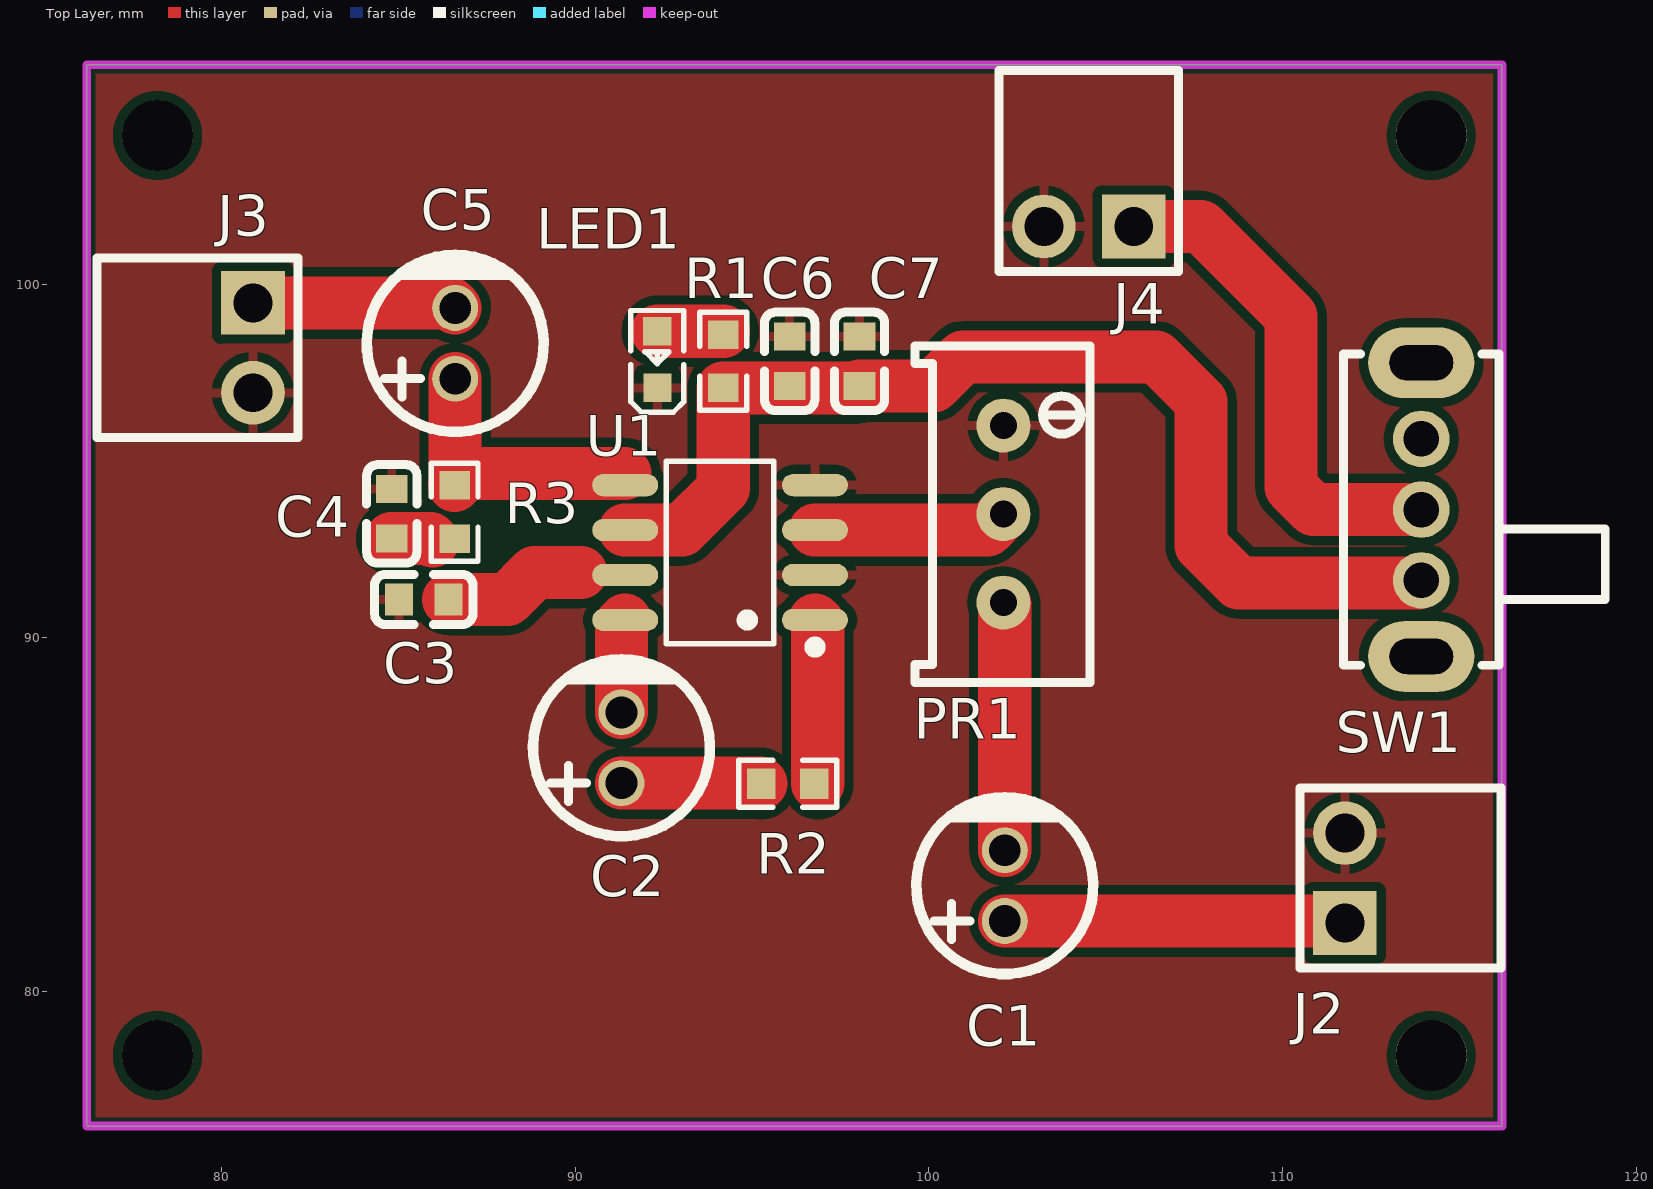
[diagram p0: Top Layer view]
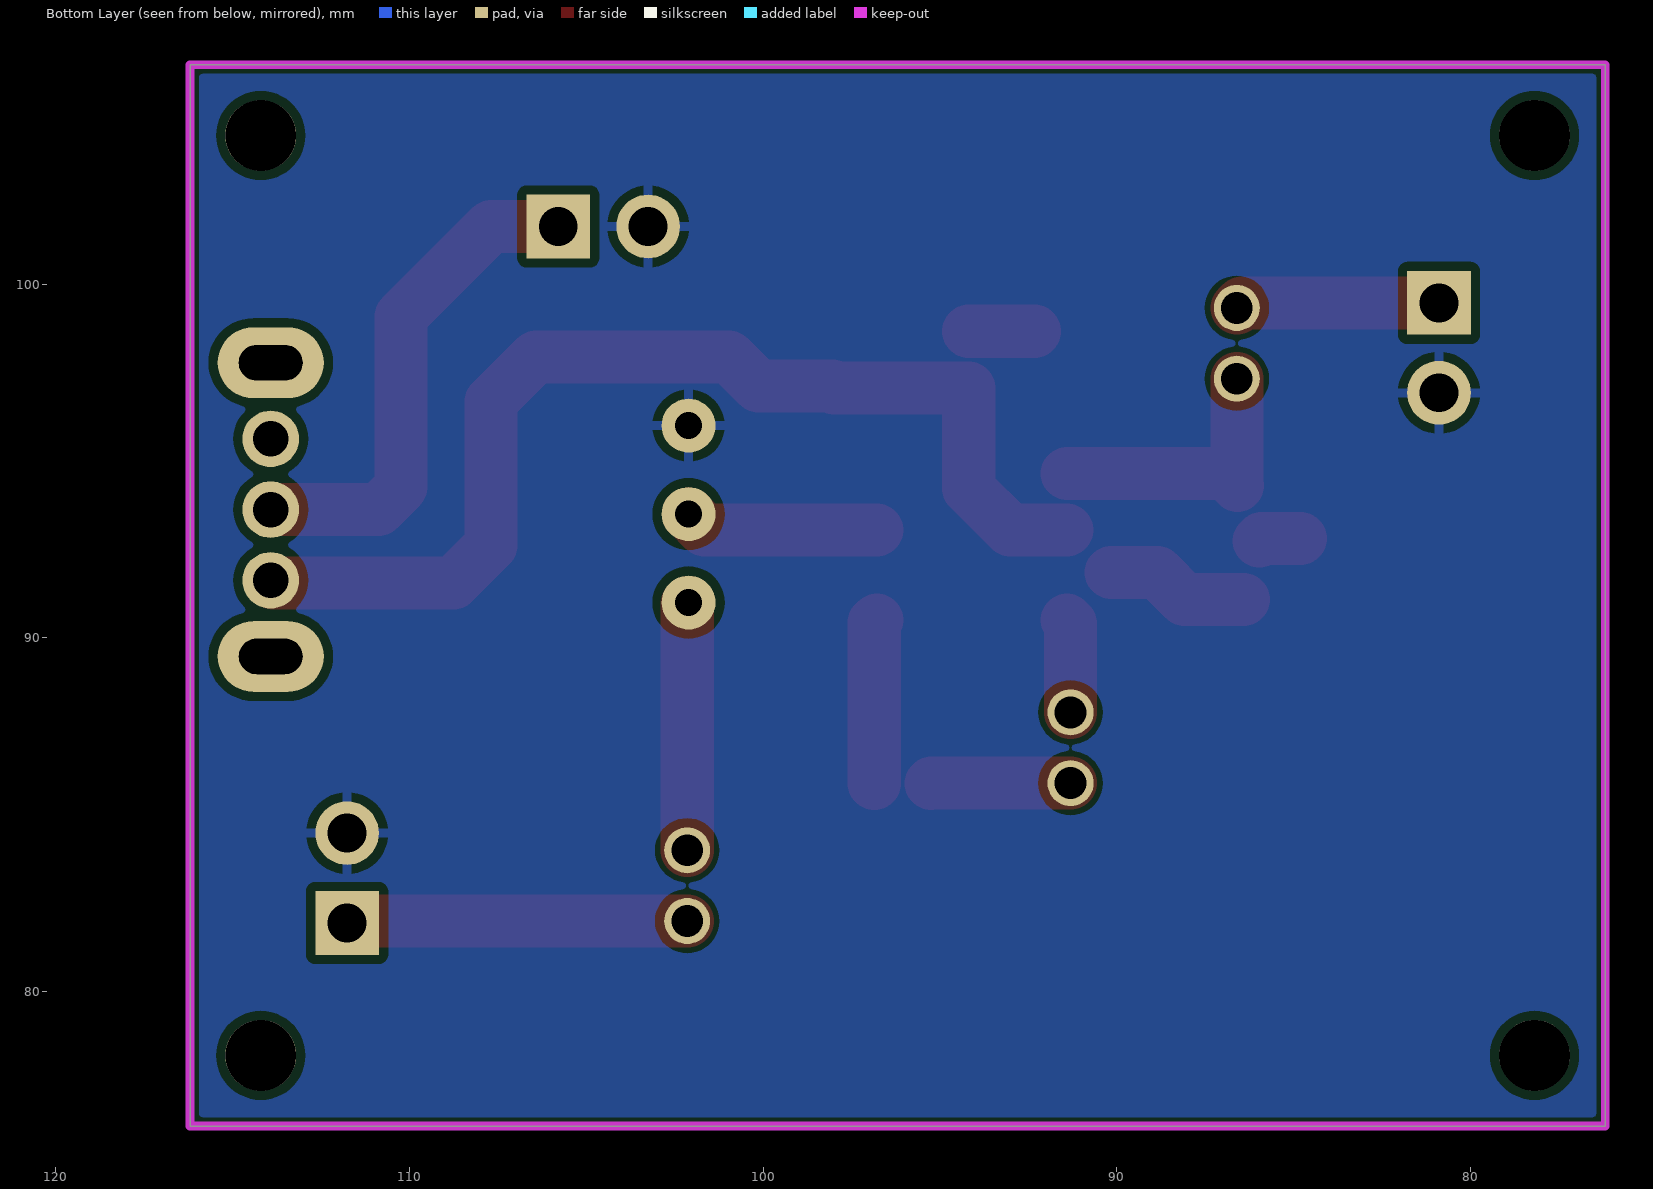
[diagram p1: Bottom Layer view, seen from below]
# Altium PCB MISC52147.pcbdoc
Units mm, origin at the board's own origin, x right, y up, seen from the top; angles counter-clockwise.
Board outline 40 x 30 mm, 2 copper layers (Top Layer, Bottom Layer), stack 1.58 mm thick; 17 components, 14 nets, 48 pads, 0 vias.

## Layer stack, top to bottom
Top Solder Mask Layer: solder mask 0.01, Dk 3.3
Top Layer: signal copper 0.035
Dielectric1: surface 1.51, FR4, Dk 4.5
Bottom Layer: signal copper 0.035
Bottom Solder Mask Layer: solder mask 0.01, Dk 3.3

## Board outline
76.2,106.2 76.2,76.2 116.2,76.2 116.2,106.2

## Design rules (kind name [scope] priority, off if disabled: settings)
BoardOutlineClearance copperThickness2oz_1 [All] p2 off: genericclearance=0.203 ignorepadtopadclearanceinfootprint=FALSE except(0: Arc-SplitContinuation Track-SplitContinuation SMDPad-SplitContinuation THPad-SplitContinuation Via-SplitContinuation Fill-SplitContinuation Region-SplitContinuation Poly-SplitContinuation Text-SplitContinuation Hole-SplitContinuation; 0.152: Arc-CutoutEdge SMDPad-CutoutEdge THPad-CutoutEdge Via-CutoutEdge Fill-CutoutEdge Region-CutoutEdge Text-CutoutEdge; 0.176: Hole-OutlineEdge Hole-CutoutEdge; 0.254: Poly-OutlineEdge Poly-CutoutEdge; 0.3: Arc-OutlineEdge Track-OutlineEdge SMDPad-OutlineEdge THPad-OutlineEdge Via-OutlineEdge Fill-OutlineEdge Region-OutlineEdge Text-OutlineEdge Track-CutoutEdge)
BoardOutlineClearance copperThickness1oz_1 [All] p4: genericclearance=0.102 ignorepadtopadclearanceinfootprint=FALSE except(0: Arc-SplitContinuation Track-SplitContinuation SMDPad-SplitContinuation THPad-SplitContinuation Via-SplitContinuation Fill-SplitContinuation Region-SplitContinuation Poly-SplitContinuation Text-SplitContinuation Hole-SplitContinuation; 0.152: SMDPad-CutoutEdge THPad-CutoutEdge Via-CutoutEdge Fill-CutoutEdge Region-CutoutEdge Text-CutoutEdge; 0.176: Hole-OutlineEdge Hole-CutoutEdge; 0.254: Poly-OutlineEdge Poly-CutoutEdge; 0.3: Arc-OutlineEdge Track-OutlineEdge SMDPad-OutlineEdge THPad-OutlineEdge Via-OutlineEdge Fill-OutlineEdge Region-OutlineEdge Text-OutlineEdge Arc-CutoutEdge Track-CutoutEdge)
Clearance copperThickness2oz [All] p1 off: gap=0.203 ignorepadtopadclearanceinfootprint=FALSE except(0.152: SMDPad-Track SMDPad-SMDPad THPad-Track SMDPad-THPad THPad-THPad Track-Via SMDPad-Via THPad-Via Via-Via Fill-Track Region-Track Fill-SMDPad Region-SMDPad Fill-THPad Region-THPad Fill-Via Region-Via Fill-Fill Fill-Region Region-Region Arc-Track Arc-SMDPad Arc-THPad Arc-Via Fill-Arc Region-Arc Arc-Arc Text-Track SMDPad-Text Text-THPad Text-Via Fill-Text Region-Text Arc-Text Text-Text; 0.176: Hole-Track Hole-SMDPad Hole-THPad Hole-Via Fill-Hole Region-Hole Hole-Arc Hole-Text; 0.254: Poly-Track Poly-SMDPad Poly-THPad Poly-Via Poly-Fill Poly-Region Poly-Poly Poly-Arc Poly-Text Poly-Hole)
Clearance copperThickness1oz [All] p3: gap=0.102 ignorepadtopadclearanceinfootprint=FALSE except(0.152: SMDPad-Track SMDPad-SMDPad THPad-Track SMDPad-THPad THPad-THPad Track-Via SMDPad-Via THPad-Via Via-Via Fill-Track Region-Track Fill-SMDPad Region-SMDPad Fill-THPad Region-THPad Fill-Via Region-Via Fill-Fill Fill-Region Region-Region Arc-Track Arc-SMDPad Arc-THPad Arc-Via Fill-Arc Region-Arc Arc-Arc Text-Track SMDPad-Text Text-THPad Text-Via Fill-Text Region-Text Arc-Text Text-Text; 0.176: Hole-Track Hole-SMDPad Hole-THPad Hole-Via Fill-Hole Region-Hole Hole-Arc Hole-Text; 0.254: Poly-Track Poly-SMDPad Poly-THPad Poly-Via Poly-Fill Poly-Region Poly-Poly Poly-Arc Poly-Text Poly-Hole)
Creepage creepage [All] p1: checkdistance=0 ignoreinternallayers=TRUE applytopolygonpour=TRUE
DiffPairsRouting differentialPair [All] p1: maxlimit=0.152 minlimit=0.152 mostfreqgap=0.152 toplayer_minwidth=0.127 toplayer_prefwidth=0.254 toplayer_maxwidth=2.54 toplayer_mingap=0.152 toplayer_prefgap=0.152 toplayer_maxgap=0.152 bottomlayer_minwidth=0.127 bottomlayer_prefwidth=0.254 bottomlayer_maxwidth=2.54 bottomlayer_mingap=0.152 bottomlayer_prefgap=0.152 bottomlayer_maxgap=0.152 maxuncoupledlength=0.254
HoleToHoleClearance otherClearance [All] p1: gap=0.3 allowstackedmicrovias=TRUE
Length netLength [All] p1: minlimit=0 maxlimit=0
MatchedLengths netLengthTolerance [All] p1: tolerance=25.4
PasteMaskExpansion pasteMaskExpansion [All] p1: expansion=0
PlaneConnect innerPlane [All] p1: planeconnectstyle=Relief reliefexpansion=0.508 reliefentries=4 reliefconductorwidth=0.254 reliefairgap=0.254
PolygonConnect copperRegion [(InNet('GND'))] p1: connectstyle=Relief reliefconductorwidth=0.254 reliefentries=4 polygonreliefangle="90 Angle" airgapwidth=0.254 via.connectstyle=Relief via.reliefconductorwidth=0.254 via.reliefentries=4 via.polygonreliefangle="90 Angle" via.airgapwidth=0.254
RoutingVias viaSize [All] p1: holewidth=0.305 width=0.61 viastyle="Through Hole" minholewidth=0.3 minwidth=0.5 maxholewidth=6.3 maxwidth=10
SolderMaskExpansion solderMaskExpansion [IsVia] p1: expansion=-25.4 istentingtop=TRUE
SolderMaskExpansion solderMaskExpansion [All] p2: expansion=0.051 istentingtop=FALSE
Width copperThickness2oz_2 [All] p1 off: maxlimit=2.54 minlimit=0.203 preferedwidth=0.254
Width copperThickness1oz_2 [All] p2: maxlimit=2.54 minlimit=0.127 preferedwidth=0.254

## Components (designator, comment, footprint, x,y, rotation, side; value= is the part's Value field where it differs from the comment)
C1 "2.2uF" CAP-TH_BD5.0-P2.00-D0.8-FD-10UF50VC110GL 102.147,82.999 r90 top
C2 "10uF" CAP-TH_BD5.0-P2.00-D0.8-FD-10UF50VC110GL 91.313,86.896 r90 top
C3 "100nF" C0603 85.725,91.087 r0 top
C4 "0.22uF" C0603 84.821,93.507 r270 top
C5 "470uF" CAP-TH_BD5.0-P2.00-D0.8-FD-10UF50VC110GL 86.614,98.326 r90 top
C6 "0.1uF" C0603 96.067,97.818 r270 top
C7 "220uF" C0603 98.044,97.818 r270 top
J2 "" HDR-TH_2P-P2.54-V-M-1 111.76,83.213 r90 top
J3 "" HDR-TH_2P-P2.54-V-M-1 80.899,98.199 r270 top
J4 "" HDR-TH_2P-P2.54-V-M-1 104.521,101.628 r180 top
LED1 "" LED_0603 92.322,97.918 r90 top
PR1 "10kΩ" R_3296 102.235,93.5 r270 top
R1 "1K" R0603 94.191,97.818 r270 top
R2 "2K2" R0603 96.012,85.88 r0 top
R3 "22E" R0603 86.599,93.557 r90 top
SW1 "" 拨动开关_侧 113.919,93.627 r90 top
U1 "LM386DTR(XBLW)" SOP-8_L4.9-W3.9-P1.27-LS6.0-BL 94.1,92.414 r90 top

## Footprints (in the part's own frame and the unit in brackets; to place one, negate y for a bottom-side part, rotate by r counter-clockwise, add the part's x,y. Pads: shape width x height; smd on the part's side, far side on the other; paste and mask are expansions set on the pad)
C0603 [mm]
  rect 0.8x0.9 smd: 1(-0.7,0) 2(0.7,0)
  silkscreen extent -1.39,-0.71 1.39,0.71
CAP-TH_BD5.0-P2.00-D0.8-FD-10UF50VC110GL [mm]
  round 1.3 hole 0.9 paste+0 mask+0.051: 1(-1,0) 2(1,0)
  silkscreen extent -2.5,-2.5 2.5,2.5
HDR-TH_2P-P2.54-V-M-1 [mm]
  rect 1.8x1.8 hole 1.1: 1(-1.27,0)
  round 1.8 hole 1.1: 2(1.27,0)
  silkscreen extent -2.54,-4.41 2.54,1.27
LED_0603 [mil]
  rect 31.5x31.5 smd paste+0 mask+2: 1(-33.5,-0.4) 2(29.5,-0.2)
  silkscreen extent -61,-30 53,30
R0603 [mm]
  rect 0.806x0.864 smd paste-100 mask+0.051: 1(-0.753,0) 2(0.753,0)
  silkscreen extent -1.39,-0.66 1.39,0.66
R_3296 [mil]
  round 60 hole 30 paste+0 mask+2: 1(-98.4,-5) 2(0,-5) 3(98.4,-5)
  silkscreen extent -187,-103 187,92
SOP-8_L4.9-W3.9-P1.27-LS6.0-BL [mm]
  oval 0.63x1.865 smd: 1(-1.905,-2.682) 2(-0.635,-2.682) 3(0.635,-2.682) 4(1.905,-2.682) 5(1.905,2.682) 6(0.635,2.682) 7(-0.635,2.682) 8(-1.905,2.682)
  silkscreen extent -2.82,-2.83 2.58,1.52
拨动开关_侧 [mil]
  round 63 hole 39.4 paste+0 mask+2: 1(-78.7,0) 2(0,0) 3(78.7,0)
  oval 78.7x118.1 hole 39.4 slot 70.9 at 90 deg paste+0 mask+2: 4(163.4,0) 5(-163.4,0)
  silkscreen extent -173,-205 173,87

## Free pads (board coordinates)
  round 2 hole 2: 1(78.2,78.2) 1(78.2,104.2) 1(114.2,78.2) 1(114.2,104.2)

## Nets (pads, with @x,y where several pads share a name; then routed paths per layer and width w, separated by ;. In a path a pad name is that pad's centre, name@x,y a point inside that pad or via, vN(x,y) a via of type N, cw(c..) or ccw(c..) an arc to the next point about the centre after c; other vN are vias at no path point)
$1N14: C1.1 J2.1 | length 9.6
  Top Layer w1.5: C1.1 111.704,81.999 J2.1
$1N15: C1.2 PR1.3 | length 7
  Top Layer w1.5: PR1.3 102.147,90.962 C1.2
$1N17: PR1.2 U1.3 | length 5.5
  Top Layer w1.5: U1.3 101.657,93.049 PR1.2
$1N20: C6.2 C7.2 R1.2 SW1.1 U1.6 | length 31.3
  Top Layer w1.5: U1.6 93.021,93.049 94.191,94.219 R1.2 97.991,97.065 C7.2 100.138,97.118 100.965,97.945 106.426,97.945 107.696,96.675 107.696,92.611 108.757,91.55 113.841,91.55 SW1.1
$1N21: LED1.2 R1.1 | length 1.9
  Top Layer w1.5: LED1.2 R1.1@94.19,98.668
$1N23: C2.2 U1.8 | length 2.7
  Top Layer w1.5: C2.2 91.313,90.404 U1.8
$1N24: C2.1 R2.1 | length 4
  Top Layer w1.5: C2.1 95.243,85.896 R2.1
$1N25: R2.2 U1.1 | length 4.7
  Top Layer w1.5: U1.1 96.861,90.43 R2.2@96.861,85.88
$1N26: C3.2 U1.7 | length 4.1
  Top Layer w1.5: C3.2 88.095,91.087 88.857,91.849 90.17,91.849
$1N29: C5.1 R3.2 U1.5 | length 8
  Top Layer w1.5: R3.2 R3.2@86.614,94.325 ; C5.1 R3.2@86.614,94.325 ; 91.417,94.651 86.939,94.651 R3.2@86.614,94.325
$1N30: C4.2 R3.1 | length 1.2
  Top Layer w1.5: C4.2 85.91,92.807 85.979,92.738
$1N33: C5.2 J3.1 | length 5.8
  Top Layer w1.5: J3.1 86.471,99.469 C5.2
$1N35: J4.1 SW1.2 | length 14.3
  Top Layer w1.5: J4.1 107.696,101.628 110.236,99.088 110.236,94.262 110.871,93.627 SW1.2
GND: C3.1 C4.1 C6.1 C7.1 J2.2 J3.2 J4.2 LED1.1 PR1.1 U1.2 U1.4
pads on no net: SW1.3 SW1.4 SW1.5

## Polygon pours and split planes (outlines as drawn)
GND on Top Layer (solid, remove dead copper, pour order 0): 76.2,106.2 76.2,76.2 116.2,76.2 116.2,106.2
GND on Bottom Layer (solid, remove dead copper, pour order 2): 76.2,106.2 76.2,76.2 116.2,76.2 116.2,106.2

## Keep-outs
Board Outline Layer:
  the board outline again, w0.254